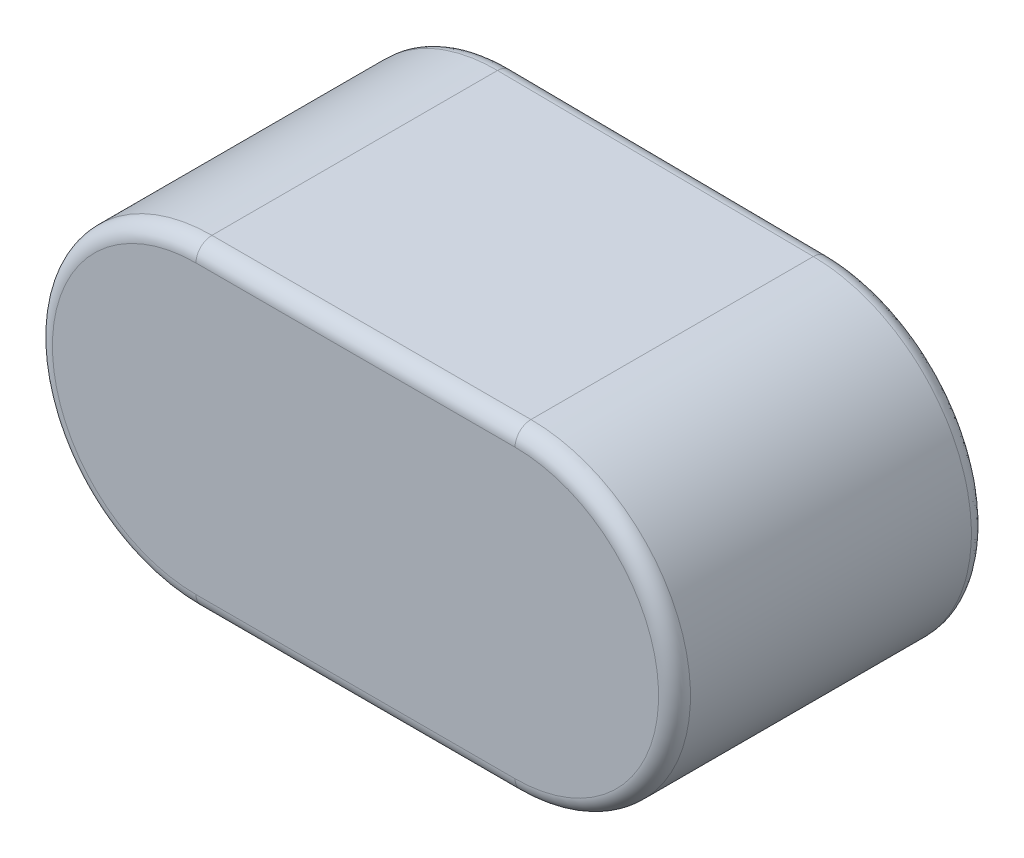
SolidWorks part; units mm, degrees
ref_plane "Front Plane" through (0, 0, 0) normal (0, 0, 1) x (1, 0, 0)
ref_plane "Top Plane" through (0, 0, 0) normal (0, 1, 0) x (1, 0, 0)
ref_plane "Right Plane" through (0, 0, 0) normal (1, 0, 0) x (0, 0, -1)
sketch "Dimension Sketch" plane through (0, 0, 0) normal (0, 0, 1) x (1, 0, 0)
  line L0 (0, 0) -> (10, 0) construction
  line L1 (0, 0) -> (0, -5) construction
  point P3 (5, 0)
  point P5 (5.25, 0)
  dimension "L" = 10
  dimension "b" = 5
  dimension "h" = 5
  dimension "r" = 0.25
sketch "Sketch1" plane through (0, 0, 0) normal (0, 0, 1) x (1, 0, 0)
  line L0 (-2.5, 2.5) -> (2.5, 2.5)
  line L1 (0, -2.5) -> (0, 2.5) construction
  line L2 (2.5, -2.5) -> (-2.5, -2.5)
  line L3 (-5, 0) -> (5, 0) construction
  arc A0 (-2.5, 2.5) -> (-2.5, -2.5) centre (-2.5, 0) ccw
  arc A1 (2.5, 2.5) -> (2.5, -2.5) centre (2.5, 0) cw
  dimension "lm" = 10
  dimension "b" = 5
extrude "Extrude1" add sketch "Sketch1" along normal blind 5
sketch "Sketch2" plane through (0, 0, 0) normal (0, 1, 0) x (1, 0, 0)
  line L0 (0, -5) -> (100, -5) construction
  line L1 (5, -5) -> (5, 0) construction
  line L4 (-5, 0) -> (5, 0)
  line L5 (5, 0) -> (5, -0.1)
  line L6 (-5, 0) -> (5, -0.1)
  line L7 (0, -5) -> (0, -4) construction
  line L8 (2.5, -5) -> (-2.5, -5) construction
  line L9 (0, -4) -> (100, -5) construction
  dimension "D1" = 100
  dimension "D2" = 1
extrude "Cut-Extrude1" cut sketch "Sketch2" against normal through all and the other way through all
fillet "Fillet2" radius 0.25 8 edges at (5, 0, 5) (0, -2.5, 5) (-5, 0, 5) (0, 2.5, 5) (-5, 0, 0) (0, 2.5, 0.05) (5, 0, 0.1) (0, -2.5, 0.05)
